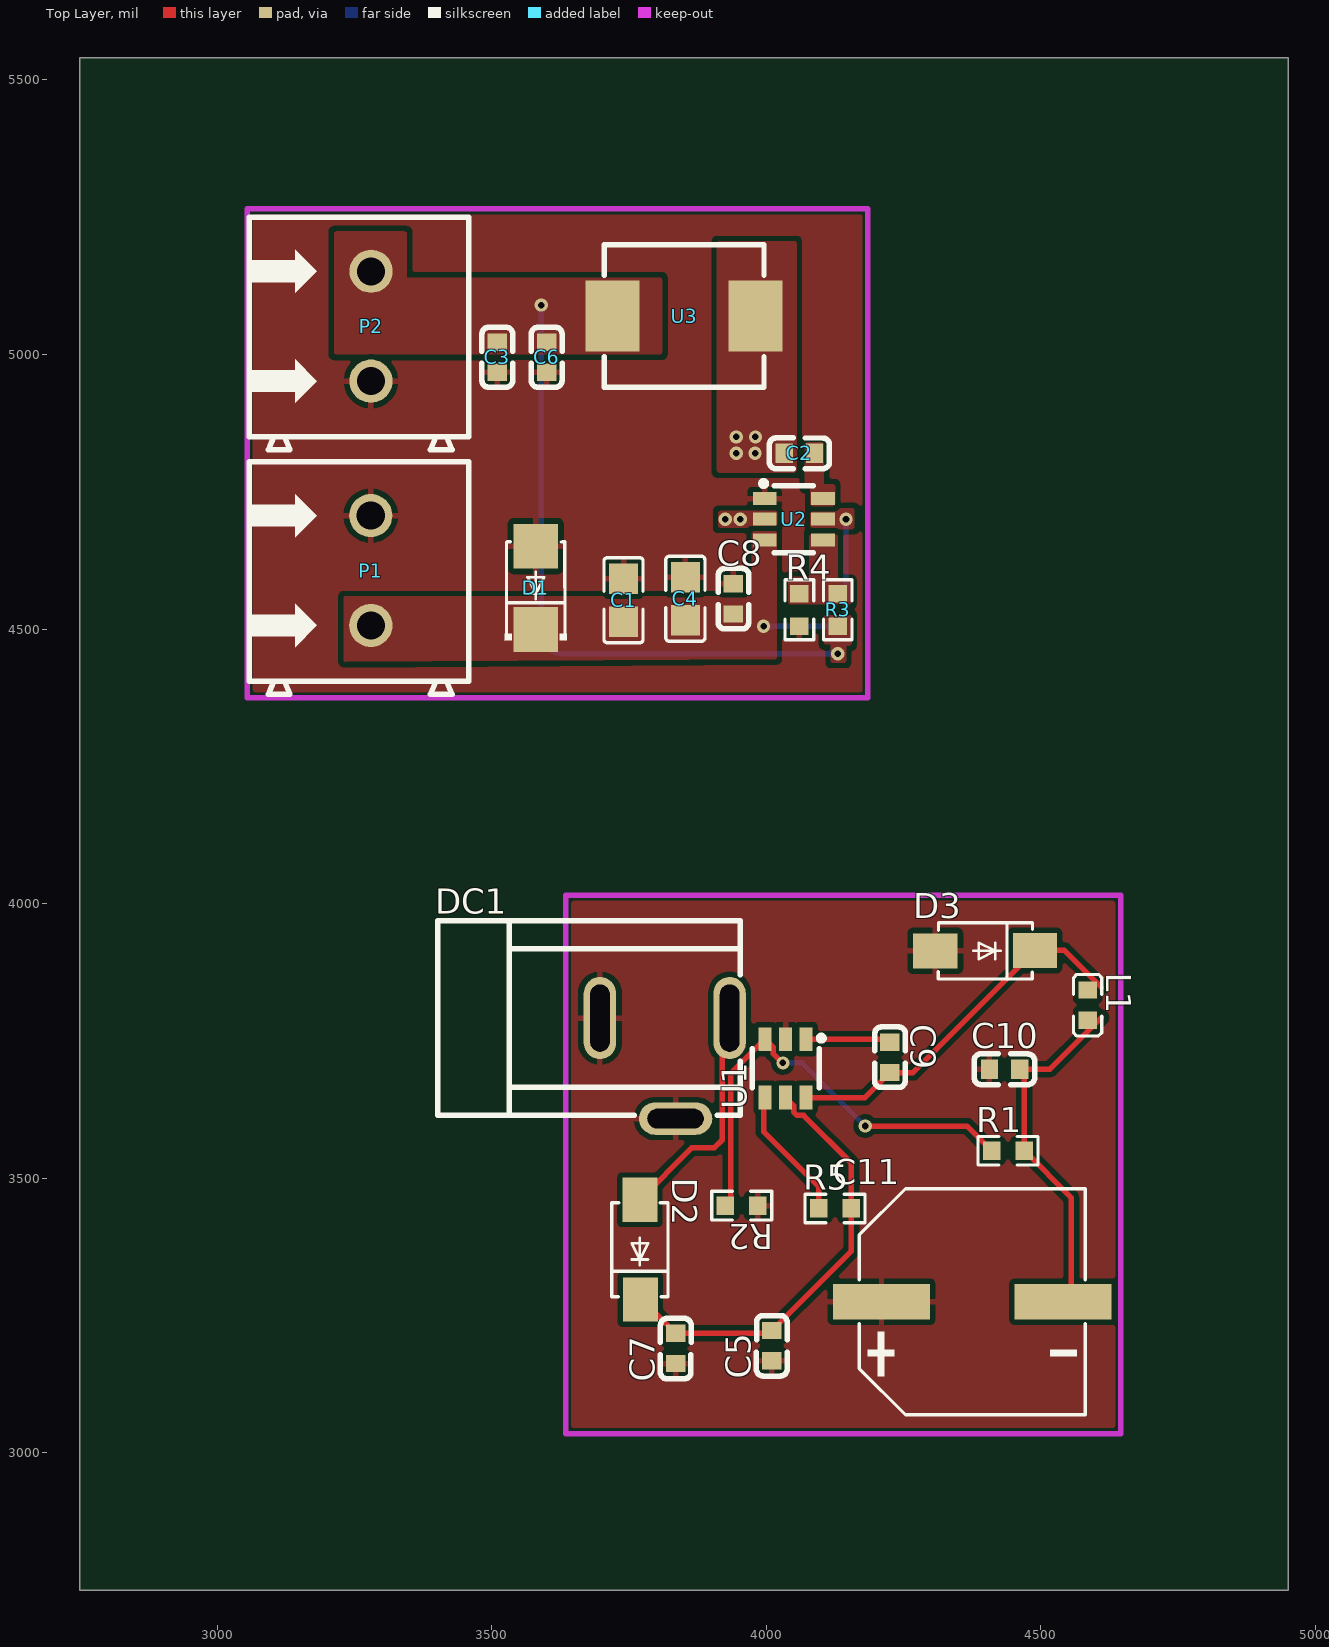
[diagram p0: Top Layer view]
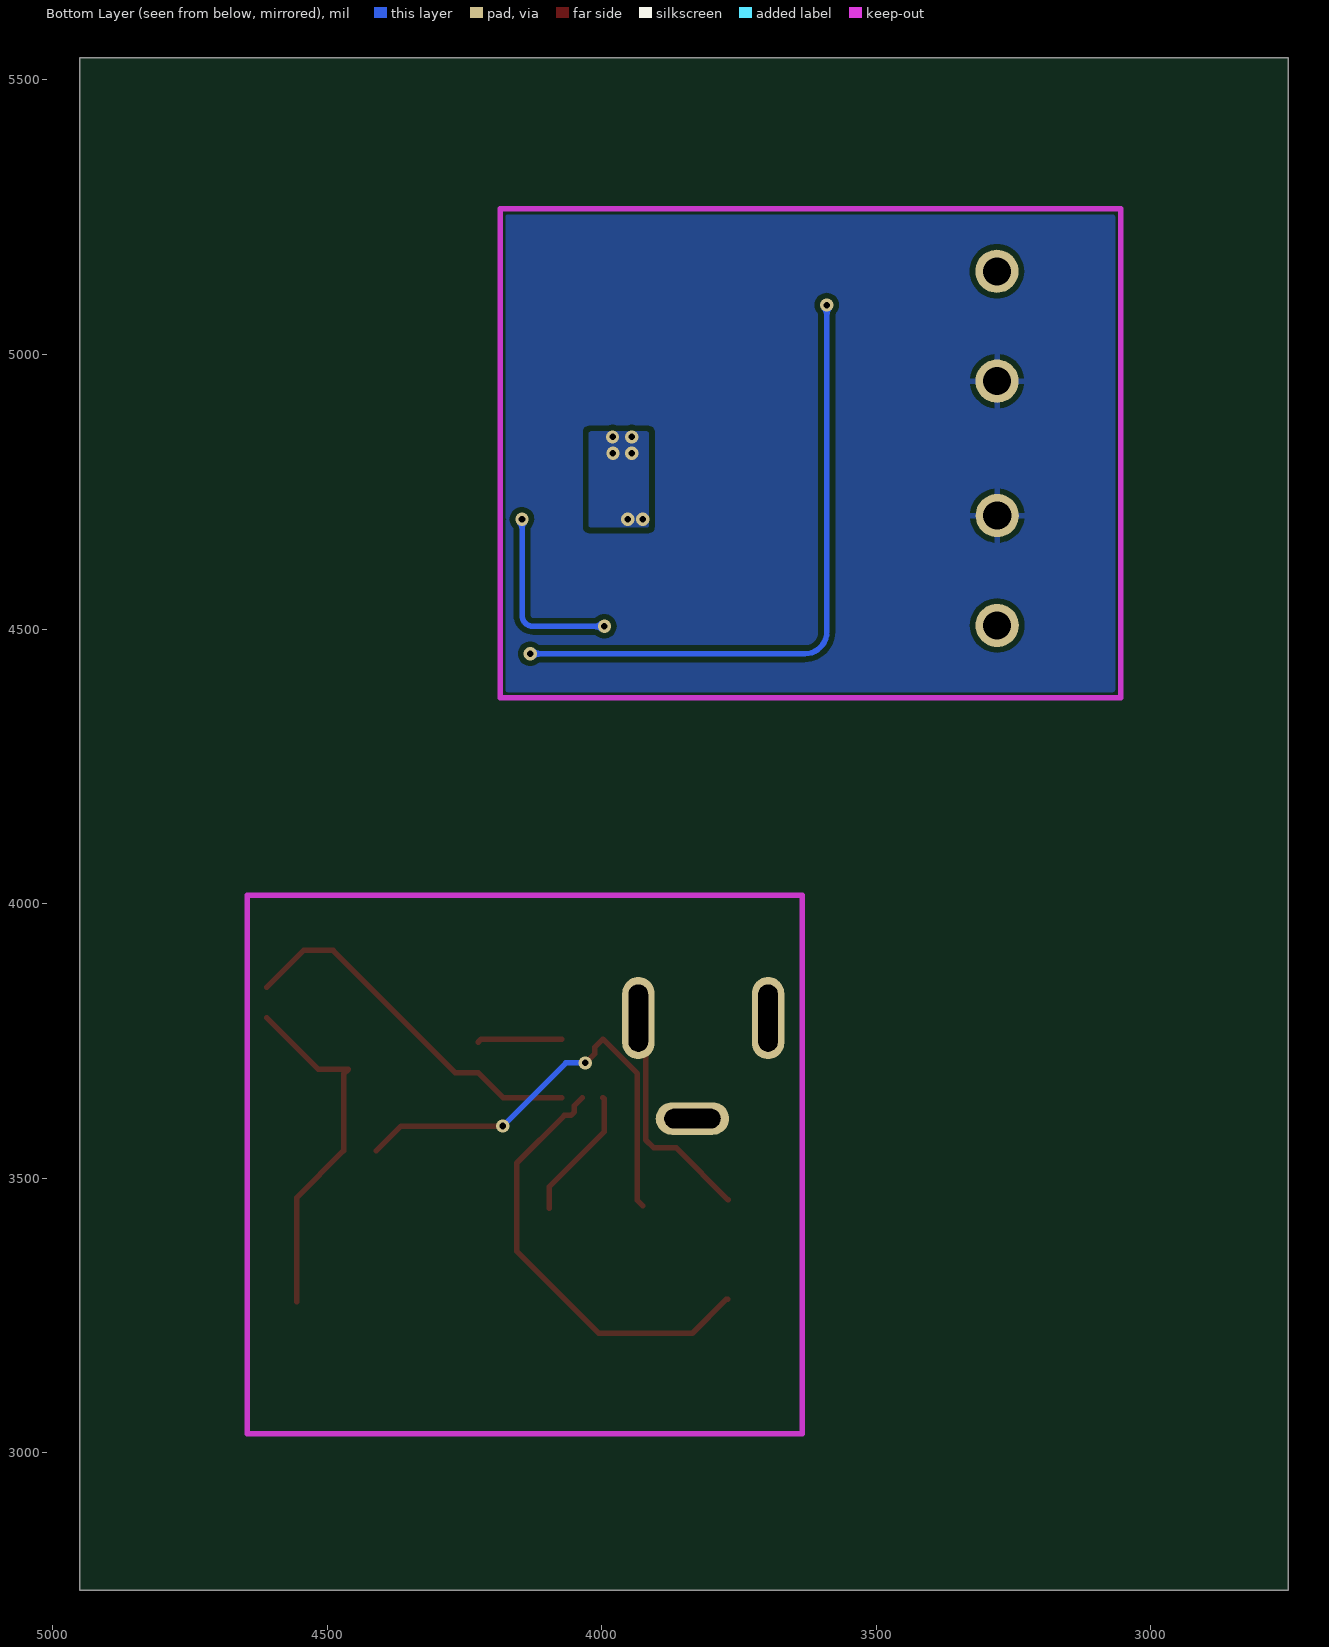
[diagram p1: Bottom Layer view, seen from below]
# Altium PCB MISC49894.pcbdoc
Units mil, origin at the board's own origin, x right, y up, seen from the top; angles counter-clockwise.
Board outline 2200 x 2790 mil, 2 copper layers (Top Layer, Bottom Layer), stack 62.206 mil thick; 26 components, 13 nets, 61 pads, 12 vias.

## Layer stack, top to bottom
Top Solder Mask Layer: solder mask 0.394, Dk 3.3
Top Layer: signal copper 1.379
DIELECTRIC1: surface 59.449, FR4, Dk 4.5
Bottom Layer: signal copper 1.378
Bottom Solder Mask Layer: solder mask 0.394, Dk 3.3

## Board outline
4950,2750 2750,2750 2750,5540 4950,5540

## Design rules (kind name [scope] priority, off if disabled: settings)
BoardOutlineClearance copperThickness2oz_1 [All] p2 off: genericclearance=7.99 ignorepadtopadclearanceinfootprint=FALSE except(0: Arc-SplitContinuation Track-SplitContinuation SMDPad-SplitContinuation THPad-SplitContinuation Via-SplitContinuation Fill-SplitContinuation Region-SplitContinuation Poly-SplitContinuation Text-SplitContinuation Hole-SplitContinuation; 5.98: Arc-CutoutEdge Track-CutoutEdge SMDPad-CutoutEdge THPad-CutoutEdge Via-CutoutEdge Text-CutoutEdge; 6.89: Hole-OutlineEdge Hole-CutoutEdge; 10: Poly-OutlineEdge Poly-CutoutEdge; 11.81: Arc-OutlineEdge Track-OutlineEdge SMDPad-OutlineEdge THPad-OutlineEdge Via-OutlineEdge Fill-OutlineEdge Region-OutlineEdge Text-OutlineEdge Fill-CutoutEdge Region-CutoutEdge)
BoardOutlineClearance Plane_innerPlane_1 [All] p4 off: genericclearance=4.02 ignorepadtopadclearanceinfootprint=FALSE except(0: Arc-SplitContinuation Track-SplitContinuation SMDPad-SplitContinuation THPad-SplitContinuation Via-SplitContinuation Fill-SplitContinuation Region-SplitContinuation Poly-SplitContinuation Text-SplitContinuation Hole-SplitContinuation; 5.98: Arc-CutoutEdge Track-CutoutEdge SMDPad-CutoutEdge THPad-CutoutEdge Via-CutoutEdge Text-CutoutEdge; 6.89: Hole-OutlineEdge Hole-CutoutEdge; 10: Poly-OutlineEdge Poly-CutoutEdge; 11.81: Arc-OutlineEdge Track-OutlineEdge SMDPad-OutlineEdge THPad-OutlineEdge Via-OutlineEdge Fill-OutlineEdge Region-OutlineEdge Text-OutlineEdge Fill-CutoutEdge Region-CutoutEdge)
BoardOutlineClearance Copper_copperRegion_1 [All] p6 off: genericclearance=4.02 ignorepadtopadclearanceinfootprint=FALSE except(0: Arc-SplitContinuation Track-SplitContinuation SMDPad-SplitContinuation THPad-SplitContinuation Via-SplitContinuation Fill-SplitContinuation Region-SplitContinuation Poly-SplitContinuation Text-SplitContinuation Hole-SplitContinuation; 5.98: Arc-CutoutEdge Track-CutoutEdge SMDPad-CutoutEdge THPad-CutoutEdge Via-CutoutEdge Text-CutoutEdge; 6.89: Hole-OutlineEdge Hole-CutoutEdge; 10: Poly-OutlineEdge Poly-CutoutEdge; 11.81: Arc-OutlineEdge Track-OutlineEdge SMDPad-OutlineEdge THPad-OutlineEdge Via-OutlineEdge Fill-OutlineEdge Region-OutlineEdge Text-OutlineEdge Fill-CutoutEdge Region-CutoutEdge)
BoardOutlineClearance Copper_copperRegion1_1 [All] p8 off: genericclearance=4.02 ignorepadtopadclearanceinfootprint=FALSE except(0: Arc-SplitContinuation Track-SplitContinuation SMDPad-SplitContinuation THPad-SplitContinuation Via-SplitContinuation Fill-SplitContinuation Region-SplitContinuation Poly-SplitContinuation Text-SplitContinuation Hole-SplitContinuation; 5.98: Arc-CutoutEdge Track-CutoutEdge SMDPad-CutoutEdge THPad-CutoutEdge Via-CutoutEdge Text-CutoutEdge; 6.89: Hole-OutlineEdge Hole-CutoutEdge; 10: Poly-OutlineEdge Poly-CutoutEdge; 11.81: Arc-OutlineEdge Track-OutlineEdge SMDPad-OutlineEdge THPad-OutlineEdge Via-OutlineEdge Fill-OutlineEdge Region-OutlineEdge Text-OutlineEdge Fill-CutoutEdge Region-CutoutEdge)
BoardOutlineClearance copperThickness1oz_1 [All] p10: genericclearance=4.02 ignorepadtopadclearanceinfootprint=FALSE except(0: Arc-SplitContinuation Track-SplitContinuation SMDPad-SplitContinuation THPad-SplitContinuation Via-SplitContinuation Fill-SplitContinuation Region-SplitContinuation Poly-SplitContinuation Text-SplitContinuation Hole-SplitContinuation; 5.98: Arc-CutoutEdge Track-CutoutEdge SMDPad-CutoutEdge THPad-CutoutEdge Via-CutoutEdge Text-CutoutEdge; 6.89: Hole-OutlineEdge Hole-CutoutEdge; 10: Poly-OutlineEdge Poly-CutoutEdge; 11.81: Arc-OutlineEdge Track-OutlineEdge SMDPad-OutlineEdge THPad-OutlineEdge Via-OutlineEdge Fill-OutlineEdge Region-OutlineEdge Text-OutlineEdge Fill-CutoutEdge Region-CutoutEdge)
Clearance copperThickness2oz [All] p1 off: gap=7.99 ignorepadtopadclearanceinfootprint=FALSE except(5.98: SMDPad-Track SMDPad-SMDPad THPad-Track SMDPad-THPad THPad-THPad Track-Via SMDPad-Via THPad-Via Via-Via Fill-SMDPad Region-SMDPad Fill-THPad Region-THPad Fill-Via Region-Via Fill-Fill Fill-Region Region-Region Arc-Track Arc-SMDPad Arc-THPad Arc-Via Fill-Arc Region-Arc Arc-Arc Text-Track SMDPad-Text Text-THPad Text-Via Fill-Text Region-Text Arc-Text Text-Text; 6.89: Hole-Track Hole-SMDPad Hole-THPad Hole-Via Fill-Hole Region-Hole Hole-Arc Hole-Text; 10: Poly-Track Poly-SMDPad Poly-THPad Poly-Via Poly-Fill Poly-Region Poly-Poly Poly-Arc Poly-Text Poly-Hole; 11.81: Fill-Track Region-Track)
Clearance Plane_innerPlane [All] p3 off: gap=4.02 ignorepadtopadclearanceinfootprint=FALSE except(5.98: SMDPad-Track SMDPad-SMDPad THPad-Track SMDPad-THPad THPad-THPad Track-Via SMDPad-Via THPad-Via Via-Via Fill-SMDPad Region-SMDPad Fill-THPad Region-THPad Fill-Via Region-Via Fill-Fill Fill-Region Region-Region Arc-Track Arc-SMDPad Arc-THPad Arc-Via Fill-Arc Region-Arc Arc-Arc Text-Track SMDPad-Text Text-THPad Text-Via Fill-Text Region-Text Arc-Text Text-Text; 6.89: Hole-Track Hole-SMDPad Hole-THPad Hole-Via Fill-Hole Region-Hole Hole-Arc Hole-Text; 10: Poly-Track Poly-SMDPad Poly-THPad Poly-Via Poly-Fill Poly-Region Poly-Poly Poly-Arc Poly-Text Poly-Hole; 11.81: Fill-Track Region-Track)
Clearance Copper_copperRegion [All] p5 off: gap=4.02 ignorepadtopadclearanceinfootprint=FALSE except(5.98: SMDPad-Track SMDPad-SMDPad THPad-Track SMDPad-THPad THPad-THPad Track-Via SMDPad-Via THPad-Via Via-Via Fill-SMDPad Region-SMDPad Fill-THPad Region-THPad Fill-Via Region-Via Fill-Fill Fill-Region Region-Region Arc-Track Arc-SMDPad Arc-THPad Arc-Via Fill-Arc Region-Arc Arc-Arc Text-Track SMDPad-Text Text-THPad Text-Via Fill-Text Region-Text Arc-Text Text-Text; 6.89: Hole-Track Hole-SMDPad Hole-THPad Hole-Via Fill-Hole Region-Hole Hole-Arc Hole-Text; 10: Poly-Track Poly-SMDPad Poly-THPad Poly-Via Poly-Fill Poly-Region Poly-Poly Poly-Arc Poly-Text Poly-Hole; 11.81: Fill-Track Region-Track)
Clearance Copper_copperRegion1 [All] p7 off: gap=4.02 ignorepadtopadclearanceinfootprint=FALSE except(5.98: SMDPad-Track SMDPad-SMDPad THPad-Track SMDPad-THPad THPad-THPad Track-Via SMDPad-Via THPad-Via Via-Via Fill-SMDPad Region-SMDPad Fill-THPad Region-THPad Fill-Via Region-Via Fill-Fill Fill-Region Region-Region Arc-Track Arc-SMDPad Arc-THPad Arc-Via Fill-Arc Region-Arc Arc-Arc Text-Track SMDPad-Text Text-THPad Text-Via Fill-Text Region-Text Arc-Text Text-Text; 6.89: Hole-Track Hole-SMDPad Hole-THPad Hole-Via Fill-Hole Region-Hole Hole-Arc Hole-Text; 10: Poly-Track Poly-SMDPad Poly-THPad Poly-Via Poly-Fill Poly-Region Poly-Poly Poly-Arc Poly-Text Poly-Hole; 11.81: Fill-Track Region-Track)
Clearance copperThickness1oz [All] p9: gap=4.02 ignorepadtopadclearanceinfootprint=FALSE except(5.98: SMDPad-Track SMDPad-SMDPad THPad-Track SMDPad-THPad THPad-THPad Track-Via SMDPad-Via THPad-Via Via-Via Fill-SMDPad Region-SMDPad Fill-THPad Region-THPad Fill-Via Region-Via Fill-Fill Fill-Region Region-Region Arc-Track Arc-SMDPad Arc-THPad Arc-Via Fill-Arc Region-Arc Arc-Arc Text-Track SMDPad-Text Text-THPad Text-Via Fill-Text Region-Text Arc-Text Text-Text; 6.89: Hole-Track Hole-SMDPad Hole-THPad Hole-Via Fill-Hole Region-Hole Hole-Arc Hole-Text; 10: Poly-Track Poly-SMDPad Poly-THPad Poly-Via Poly-Fill Poly-Region Poly-Poly Poly-Arc Poly-Text Poly-Hole; 11.81: Fill-Track Region-Track)
DiffPairsRouting differentialPair [All] p1: maxlimit=6 minlimit=6 mostfreqgap=6 toplayer_minwidth=5 toplayer_prefwidth=10 toplayer_maxwidth=100 toplayer_mingap=6 toplayer_prefgap=6 toplayer_maxgap=6 bottomlayer_minwidth=5 bottomlayer_prefwidth=10 bottomlayer_maxwidth=100 bottomlayer_mingap=6 bottomlayer_prefgap=6 bottomlayer_maxgap=6 maxuncoupledlength=10
HoleToHoleClearance otherClearance [All] p1: gap=11.81 allowstackedmicrovias=TRUE
Length netLength [All] p1: minlimit=0 maxlimit=0
PasteMaskExpansion pasteMaskExpansion [All] p1: expansion=0
PlaneConnect innerPlane [All] p1: planeconnectstyle=Relief reliefexpansion=20 reliefentries=4 reliefconductorwidth=10 reliefairgap=10
PolygonConnect copperRegion1 [All] p1 off: connectstyle=Direct reliefconductorwidth=10 reliefentries=4 polygonreliefangle="90 Angle" airgapwidth=10 via.connectstyle=Relief via.reliefconductorwidth=10 via.reliefentries=4 via.polygonreliefangle="90 Angle" via.airgapwidth=10
PolygonConnect copperRegion [All] p2: connectstyle=Relief reliefconductorwidth=10 reliefentries=4 polygonreliefangle="90 Angle" airgapwidth=10 via.connectstyle=Relief via.reliefconductorwidth=10 via.reliefentries=4 via.polygonreliefangle="90 Angle" via.airgapwidth=10
RoutingVias viaSize [All] p1: holewidth=12.01 width=24.02 viastyle="Through Hole" minholewidth=11.81 minwidth=19.68 maxholewidth=248.03 maxwidth=393.7
SolderMaskExpansion solderMaskExpansion [IsVia] p1: expansion=-1000 istentingtop=TRUE
SolderMaskExpansion solderMaskExpansion [All] p2: expansion=2.01 istentingtop=FALSE
Width copperThickness2oz_2 [All] p1 off: maxlimit=100 minlimit=8 preferedwidth=10
Width copperThickness1oz_2 [All] p2: maxlimit=100 minlimit=5 preferedwidth=10

## Components (designator, comment, footprint, x,y, rotation, side; value= is the part's Value field where it differs from the comment)
C1 "10uF" C0805 3739.9,4552.5 r270 top
C2 "100nF" C0603 4060,4820 r0 top
C3 "22uF" C0603 3510,4995 r90 top
C4 "10uF" C0805 3852.5,4555.1 r270 top
C5 "10uF" C0603 4010,3195 r90 top
C6 "22uF" C0603 3600,4995 r90 top
C7 "100nF" C0603 3835,3190 r90 top
C8 "100nF" C0603 3940,4555 r270 top
C9 "100nF" C0603 4225,3720 r270 top
C10 "100nF" C0603 4433.77,3698.33 r0 top
C11 "220uF" CAP-SMD_BD10.0-L10.3-W10.3-LS11.7-FD 4375,3275 r0 top
D1 "SMAJ12A" DO-214AC_L4.3-W2.7-LS5.0-RD 3580,4575 r90 top
D2 "SS14" SMA_L4.3-W2.6-LS5.0-FD 3770,3370 r270 top
D3 "SS14" SMA_L4.3-W2.6-LS5.0-FD 4398.39,3914.35 r0 top
DC1 "DC-005-A200" DC-IN-TH_DC-005-A200 3815,3700 r0 top
L1 "4.7uH" L0603 4585,3815 r270 top
P1 "WJ500V-5.08-2P" CONN-TH_2P-P5.00_WJ500V-5.08-2P#1 3280,4605 r90 top
P2 "WJ500V-5.08-2P" CONN-TH_2P-P5.00_WJ500V-5.08-2P#2 3280,5050 r90 top
R1 "49.9kΩ" R0603 4440,3550 r0 top
R2 "9.53kΩ" R0603 3955,3450 r180 top
R3 "53.6kΩ" R0603 4130,4535 r270 top
R4 "10kΩ" R0603 4060,4535 r90 top
R5 "100kΩ" R0603 4125,3445 r0 top
U1 "MP2359DT-LF-Z" SOT-23-6_L2.9-W1.6-P0.95-LS2.8-BR 4035,3700 r90 top
U2 "TPS563201DDCR" SOT-23-6_L2.9-W1.6-P0.95-LS2.8-BR 4050,4700 r180 top
U3 "3.3uH" IND-SMD_L7.4-W6.6 3850,5070 r180 top

## Footprints (in the part's own frame and the unit in brackets; to place one, negate y for a bottom-side part, rotate by r counter-clockwise, add the part's x,y. Pads: shape width x height; smd on the part's side, far side on the other; paste and mask are expansions set on the pad)
C0603 [mm]
  rect 0.8x0.9 smd: 1(-0.7,0) 2(0.7,0)
  silkscreen extent -1.39,-0.71 1.39,0.71
C0805 [mm]
  rect 1.41x1.35 smd paste-100 mask+0.051: 1(-1,0) 2(1,0)
  silkscreen extent -1.96,-0.9 1.96,0.9
CAP-SMD_BD10.0-L10.3-W10.3-LS11.7-FD [mm]
  rect 4.5x1.65 smd: 1(-4.2,0) 2(4.2,0)
  silkscreen extent -5.23,-5.23 5.23,5.23
CONN-TH_2P-P5.00_WJ500V-5.08-2P#1 [mm]
  round 2 hole 1.3: 1(2.581,0.011) 2(-2.502,0.007)
  silkscreen extent -5.68,-4.52 5.08,5.64
CONN-TH_2P-P5.00_WJ500V-5.08-2P#2 [mm]
  round 2 hole 1.3: 1(2.578,-0.005) 2(-2.503,0.001)
  silkscreen extent -5.68,-4.52 5.08,5.64
DC-IN-TH_DC-005-A200 [mm]
  oval 1.5x3.8 hole 0.9 slot 3.1 at 90 deg copper offset -0.001,0: 1(3.001,2.325)
  oval 1.5x3.8 hole 0.9 slot 3.1 at 90 deg copper offset 0,0: 2(-3,2.325)
  oval 3.4x1.5 hole 0.9 slot 2.6 at 0 deg copper offset 0,-0.001: 3(0.5,-2.325)
  silkscreen extent -10.5,-2.17 3.5,6.83
DO-214AC_L4.3-W2.7-LS5.0-RD [mm]
  rect 2.07x2.06 smd: 1(-1.929,0) 2(1.929,0)
  silkscreen extent -2.43,-1.43 2.14,1.43
IND-SMD_L7.4-W6.6 [mm]
  rect 2.5x3.3 smd: 1(-3.302,0) 2(3.302,0)
  silkscreen extent -3.7,-3.3 3.7,3.3
L0603 [mm]
  rect 0.8x0.864 smd paste-100 mask+0.051: 1(-0.7,0) 2(0.7,0)
  silkscreen extent -1.42,-0.65 1.42,0.65
R0603 [mil]
  rect 31.75x34.02 smd paste-3937.01 mask+2: 1(-29.66,0) 2(29.66,0)
  silkscreen extent -55,-26 55,26
SMA_L4.3-W2.6-LS5.0-FD [mm]
  rect 2.046x1.62 smd: 1(-2.304,-0.009) 2(2.304,0.009)
  silkscreen extent -2.17,-1.32 2.19,1.29
SOT-23-6_L2.9-W1.6-P0.95-LS2.8-BR [mm]
  rect 1.1x0.6 smd paste+0 mask+0.051: 1(1.35,-0.95) 2(1.35,0) 3(1.35,0.95) 4(-1.35,0.95) 5(-1.35,0) 6(-1.35,-0.95)
  silkscreen extent -0.9,-1.78 1.52,1.55

## Via types
v1: diameter 24.02, hole 12, Top Layer to Bottom Layer, 12 vias

## Nets (pads, with @x,y where several pads share a name; then routed paths per layer and width w, separated by ;. In a path a pad name is that pad's centre, name@x,y a point inside that pad or via, vN(x,y) a via of type N, cw(c..) or ccw(c..) an arc to the next point about the centre after c; other vN are vias at no path point)
$1N3448: R3.1 R4.2 U2.4
$1N3766: C2.2 U2.6
$1N3805: C2.1 U2.2 U3.1
  other v1: 3925,4700 3952.38,4700 3945,4820 3979.47,4820 3945,4850 3980,4850
$1N4312: D2.1 DC1.1 | length 422.6
  Top Layer w10: D2.1 3863.93,3555 3905,3555 3920,3570 3920,3778.43 DC1.1
$1N4314: C9.1 U1.1 | length 154.9
  Top Layer w10: U1.1 4219.41,3753.15 C9.1
$1N4319: C5.2 C7.2 D2.2 R5.2 U1.5 | length 807.8
  Top Layer w10: D2.2 3773.26,3279.3 C7.2 4005,3217.56 C5.2 4154.66,3367.22 R5.2 4154.66,3527.19 4067.64,3614.21 4056.04,3614.21 4049.6,3620.65 4049.6,3632.25 U1.5
$1N4323: R5.1 U1.4 | length 244.5
  Top Layer w10: U1.4 3995,3644.25 3995,3585 4095.34,3484.66 R5.1
$1N4324: R1.1 R2.2 U1.3 | length 836.8
  Top Layer w10: R2.2 3935,3459.66 3935,3690.55 U1.3 4012.2,3738.55 4012.2,3726.95 4029.15,3710 v1(4030,3710) ; v1(4180,3595) 4365.34,3595 R1.1
  Bottom Layer w10: v1(4030,3710) 4065,3710 v1(4180,3595)
$1N4327: C9.2 D3.2 L1.1 U1.6 | length 676.4
  Top Layer w10: U1.6 4179.41,3646.85 C9.2 4266.82,3692.44 D3.2 4542.84,3914.72 4610,3847.55
+5V: C3.2 C6.2 P2.1 R3.2 U3.2 | length 1157.8
  Bottom Layer w10: v1(3590,5090) 3590,4495 ccw(c3630,4495) 3630,4455 v1(4130,4455)
+12V: C1.2 C4.2 C8.2 D1.1 P1.2 U2.3 U2.5 | length 336.4
  Bottom Layer w10: v1(3995,4505) 4125,4505 ccw(c4125,4525) 4145,4525 v1(4145,4700)
GND: C1.1 C3.1 C4.1 C5.1 C6.1 C7.1 C8.1 C10.1 C11.1 D1.2 D3.1 DC1.2 DC1.3 P1.1 P2.2 R2.1 R4.1 U1.2 U2.1
VOUT: C10.2 C11.2 L1.2 R1.2 | length 649.9
  Top Layer w10: C11.2@4555.35,3275 4555.35,3464.3 R1.2 4469.66,3689.99 C10.2 4515.88,3698.33 4610,3792.45

## Polygon pours and split planes (outlines as drawn)
$1N3805 on Top Layer (solid, remove dead copper, pour order 2): 3910,4785 4055,4785 4055,5206.48 3910,5206.48
$1N3766 on Top Layer (solid, remove dead copper, pour order 8): 4070,4840 4070,4757.09 4072.91,4760 4080,4760 4080,4723.86 4123.86,4723.86 4125,4725 4125,4763.97 4104.87,4763.97 4104.87,4840
+12V on Top Layer (solid, remove dead copper, pour order 10): 4080,4720 4080,4682.09 4160,4682.09 4160,4720.06 4080.06,4720.06
$1N3805 on Top Layer (solid, remove dead copper, pour order 4): 4020,4685 4020,4715 3912.41,4715 3912.41,4684.37 4019.37,4684.37
$1N3805 on Bottom Layer (solid, remove dead copper, pour order 20): 3913.86,4685 4023.5,4685 4023.5,4860 3913.75,4860 3913.75,4686.25
+5V on Top Layer (solid, remove dead copper, pour order 12): 4105,4525 4155.3,4525 4155.3,4470 4145,4470 4145,4438.58 4117.12,4438.58 4117.12,4471.96 4105,4471.96
$1N3448 on Top Layer (solid, remove dead copper, pour order 14): 4040,4545 4155,4545 4155,4589.55 4130,4590 4130,4675.06 4077.86,4675.06 4077.86,4595 4040,4595
+12V on Top Layer (solid, remove dead copper, pour order 0): 3230,4560 3973.66,4560 3973.66,4678.11 4019.22,4678.11 4019.22,4445.16 3230,4440.03
GND on Top Layer (solid, pour order 16): 3000,5290 3000,4350 4215,4350 4215,5290
+5V on Top Layer (solid, remove dead copper, pour order 6): 3810,5000 3810,5140 3345,5140 3345,5224.02 3213.07,5224.02 3213.07,5000
GND on Bottom Layer (solid, pour order 22): 3000,5290 3000,4350 4215,4350 4215,5290
GND on Top Layer (solid, remove dead copper, pour order 18): 3565,4070 3565,3000 4700,3000 4700,4070

## Keep-outs
Board Outline Layer:
  lines w10: 3055,4375 3055,5265 4185,5265 4185,4375 3055,4375 ; 3635,3035 3635,4015 4645,4015 4645,3035 3635,3035

## Other copper
Bottom Layer:
  region net +12V: 4150,4683.59 4140,4683.59 4139.91,4684.71 4139.66,4685.84 4138.77,4688.07 4137.5,4690.17 4136.05,4691.99 4153.95,4691.99 4152.5,4690.17 4151.23,4688.07 4150.34,4685.84 4150.09,4684.71
  region net +12V: 4011.41,4510 4011.41,4500 4010.29,4499.91 4009.16,4499.66 4006.93,4498.77 4004.83,4497.5 4003.01,4496.05 4003.01,4513.95 4004.83,4512.5 4006.93,4511.23 4009.16,4510.34 4010.29,4510.09
  region net +5V: 4113.59,4450 4113.59,4460 4114.71,4460.09 4115.84,4460.34 4118.07,4461.23 4120.17,4462.5 4121.99,4463.95 4121.99,4446.05 4120.17,4447.5 4118.07,4448.77 4115.84,4449.66 4114.71,4449.91
  region net +5V: 3595,5073.59 3585,5073.59 3584.91,5074.71 3584.66,5075.84 3583.77,5078.07 3582.5,5080.17 3581.05,5081.99 3598.95,5081.99 3597.5,5080.17 3596.23,5078.07 3595.34,5075.84 3595.09,5074.71